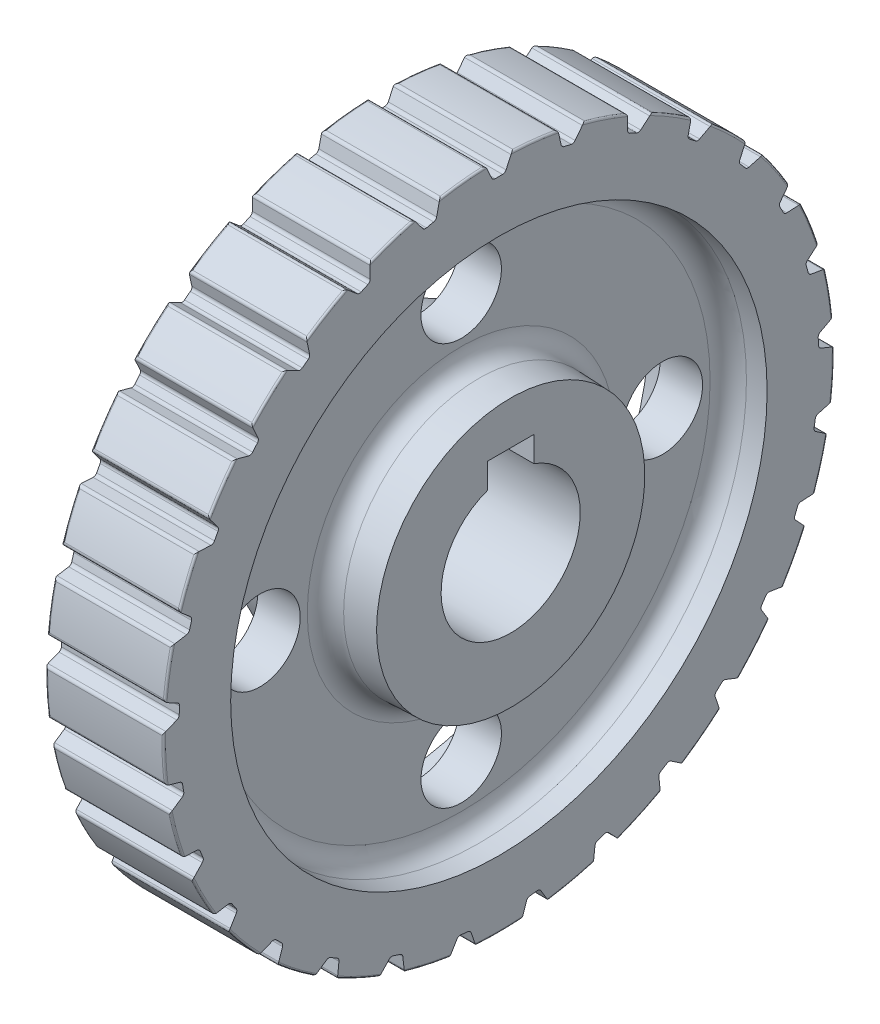
from build123d import *

# Parameters (mm, degrees)
CHAMFER1_SIZE       = 1
SKETCH4_W           = 5
SKETCH4_H           = 2.746034567
CUT_EXTRUDE1_DEPTH  = 54.34158084
FILLET1_R           = 2
SKETCH5_R           = 4.33752
CUT_EXTRUDE2_DEPTH  = 53.992712201
CIRPATTERN1_COUNT   = 4
CUT_EXTRUDE3_REACH  = 54.993
CIRPATTERN3_COUNT   = 29
SKETCH9_R           = 12.5
BOSS_EXTRUDE3_DEPTH = 15.24
CUT_EXTRUDE5_DEPTH  = 54.34158084


with BuildPart() as part:
    # Sketch1 → Revolve1 (revolve)
    with BuildSketch(Plane.XY, mode=Mode.PRIVATE) as revolve1_sk:
        with BuildLine():
            Line((-1.27, 7.2292), (-1.27, 14.4584))
            Line((-1.27, 14.4584), (4.064, 14.671703117))
            Line((4.064, 14.671703117), (4.064, 28.75428334))
            Line((4.064, 28.75428334), (0, 28.9168))
            Line((0, 28.9168), (0, 35.946))
            ThreePointArc((0, 35.946), (0.058578644, 36.087421356), (0.2, 36.146))
            Line((0.2, 36.146), (12.5, 36.146))
            ThreePointArc((12.5, 36.146), (12.641421356, 36.087421356), (12.7, 35.946))
            Line((12.7, 35.946), (12.7, 28.9168))
            Line((12.7, 28.9168), (8.636, 28.75428334))
            Line((8.636, 28.75428334), (8.636, 14.671703117))
            Line((8.636, 14.671703117), (13.97, 14.4584))
            Line((13.97, 14.4584), (13.97, 7.2292))
            Line((13.97, 7.2292), (-1.27, 7.2292))
        make_face()
    revolve(revolve1_sk.sketch.rotate(Axis((0, 0, 0), (1, 0, 0)), 90), axis=Axis((0, 0, 0), (1, 0, 0)))

    # Chamfer1
    chamfer1_edges = [part.edges().sort_by_distance(p)[0] for p in [
        (-1.27, 0, -7.2292),
        (13.97, 0, -7.2292),
    ]]
    chamfer(chamfer1_edges, length=CHAMFER1_SIZE)

    # Sketch4 → Cut-Extrude1 (cut, through all)
    with BuildSketch(Plane.ZY.offset(1.27)):
        with Locations((0, 8.156182669)):
            Rectangle(SKETCH4_W, SKETCH4_H)
    extrude(amount=-CUT_EXTRUDE1_DEPTH, mode=Mode.SUBTRACT)

    # Fillet1
    fillet1_edges = [part.edges().sort_by_distance(p)[0] for p in [
        (8.636, 0, -14.671703117),
        (8.636, 0, -28.75428334),
        (4.064, 0, -28.75428334),
        (4.064, 0, -14.671703117),
    ]]
    fillet(fillet1_edges, radius=FILLET1_R)

    # Sketch5 → Cut-Extrude2 (cut, through all)
    with BuildSketch(Plane(origin=(0, 0, 0), x_dir=(0, 0, -1), z_dir=(1, 0, 0))):
        with Locations(Location((0, 21.6876, 0), (0, 0, 180))):
            Circle(SKETCH5_R)
    cut_extrude2 = extrude(amount=CUT_EXTRUDE2_DEPTH, mode=Mode.SUBTRACT)

    # CirPattern1: Cut-Extrude2 ×4 about axis
    cirpattern1_axis = Axis((0, 0, 0), (1, 0, 0))
    for i in range(1, CIRPATTERN1_COUNT):
        add(cut_extrude2.rotate(cirpattern1_axis, i * 360 / CIRPATTERN1_COUNT), mode=Mode.SUBTRACT)

    # Sketch6 → Cut-Extrude3 (cut, up to next)
    with BuildSketch(Plane(origin=(0, 0, 0), x_dir=(0, 0, -1), z_dir=(1, 0, 0)), mode=Mode.PRIVATE) as cut_extrude3_sk1:
        with BuildLine():
            Line((-1.312143604, 35.888212119), (-0.772259465, 34.730426846))
            ThreePointArc((-0.772259465, 34.730426846), (-0.618977849, 34.556651184), (-0.395967031, 34.493727344))
            ThreePointArc((-0.395967031, 34.493727344), (0, 34.496), (0.395967031, 34.493727344))
            ThreePointArc((0.395967031, 34.493727344), (0.618977849, 34.556651184), (0.772259465, 34.730426846))
            Line((0.772259465, 34.730426846), (1.312143604, 35.888212119))
            ThreePointArc((1.312143604, 35.888212119), (1.459845379, 36.052749468), (1.67414067, 36.107209377))
            ThreePointArc((1.67414067, 36.107209377), (1.86391364, 36.097910493), (2.053635109, 36.087614203))
            Line((2.053635109, 36.087614203), (17.485587767, 69.181543475))
            ThreePointArc((17.485587767, 69.181543475), (0, 71.357072089), (-17.485587767, 69.181543475))
            Line((-17.485587767, 69.181543475), (-2.053635109, 36.087614203))
            ThreePointArc((-2.053635109, 36.087614203), (-1.86391364, 36.097910493), (-1.67414067, 36.107209377))
            ThreePointArc((-1.67414067, 36.107209377), (-1.459845379, 36.052749468), (-1.312143604, 35.888212119))
        make_face()
    cut_extrude3_tool1 = extrude(cut_extrude3_sk1.sketch, amount=CUT_EXTRUDE3_REACH, mode=Mode.PRIVATE) & part.part
    cut_extrude3 = cut_extrude3_tool1.solids().sort_by_distance((0, 57.83829, 0))[0]
    add(cut_extrude3, mode=Mode.SUBTRACT)

    # CirPattern3: Cut-Extrude3 ×29 about axis
    cirpattern3_axis = Axis((0, 0, 0), (1, 0, 0))
    for i in range(1, CIRPATTERN3_COUNT):
        add(cut_extrude3.rotate(cirpattern3_axis, i * 360 / CIRPATTERN3_COUNT), mode=Mode.SUBTRACT)

    # Sketch9 → Boss-Extrude3 (add)
    with BuildSketch(Plane.ZY.offset(1.27)):
        Circle(SKETCH9_R)
    extrude(amount=-BOSS_EXTRUDE3_DEPTH)

    # Sketch10 → Cut-Extrude5 (cut, through all)
    with BuildSketch(Plane.ZY.offset(1.27)):
        with BuildLine():
            Line((-2.5, 7.071067812), (-2.5, 9.8))
            Line((-2.5, 9.8), (2.5, 9.8))
            Line((2.5, 9.8), (2.5, 7.071067812))
            ThreePointArc((2.5, 7.071067812), (0, -7.5), (-2.5, 7.071067812))
        make_face()
    extrude(amount=-CUT_EXTRUDE5_DEPTH, mode=Mode.SUBTRACT)


solid = part.part
